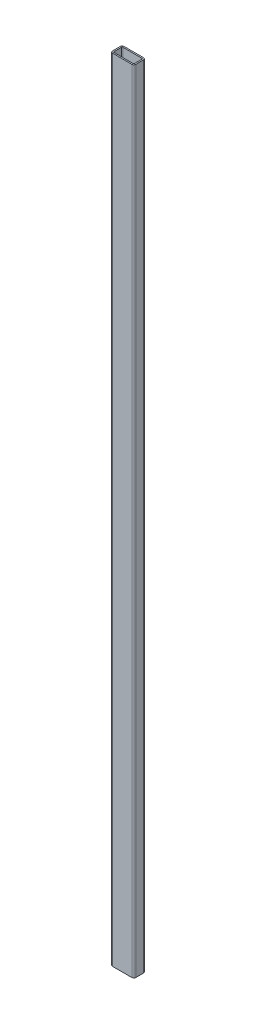
SolidWorks part; units mm, degrees
ref_plane "Front" through (0, 0, 0) normal (0, 0, 1) x (1, 0, 0)
ref_plane "Top" through (0, 0, 0) normal (0, 1, 0) x (1, 0, 0)
ref_plane "Right" through (0, 0, 0) normal (1, 0, 0) x (0, 0, -1)
sketch "Sketch1" plane through (0, 0, 0) normal (0, 1, 0) x (1, 0, 0)
  line L0 (-16.55, -7.7) -> (16.55, -7.7)
  line L1 (-16.55, -10) -> (16.55, -10)
  line L2 (-20, -6.55) -> (-20, 6.55)
  line L3 (-16.55, 10) -> (16.55, 10)
  line L4 (20, -6.55) -> (20, 6.55)
  line L5 (-20, -10) -> (20, 10) construction
  line L6 (-20, 10) -> (20, -10) construction
  line L7 (17.7, -6.55) -> (17.7, 6.55)
  line L8 (-16.55, 7.7) -> (16.55, 7.7)
  line L9 (-17.7, -6.55) -> (-17.7, 6.55)
  arc A0 (16.55, 10) -> (20, 6.55) centre (16.55, 6.55) cw
  arc A1 (-16.55, -10) -> (-20, -6.55) centre (-16.55, -6.55) cw
  arc A2 (16.55, -10) -> (20, -6.55) centre (16.55, -6.55) ccw
  arc A3 (-20, 6.55) -> (-16.55, 10) centre (-16.55, 6.55) cw
  arc A4 (16.55, -7.7) -> (17.7, -6.55) centre (16.55, -6.55) ccw
  arc A5 (16.55, 7.7) -> (17.7, 6.55) centre (16.55, 6.55) cw
  arc A6 (-17.7, 6.55) -> (-16.55, 7.7) centre (-16.55, 6.55) cw
  arc A7 (-16.55, -7.7) -> (-17.7, -6.55) centre (-16.55, -6.55) cw
  point P0 (0, 0)
  dimension "D3" = 3.45
  dimension "D1" = 40
  dimension "D2" = 20
  dimension "D4" = 2.3
extrude "Boss-Extrude1" add sketch "Sketch1" along normal blind 1360
